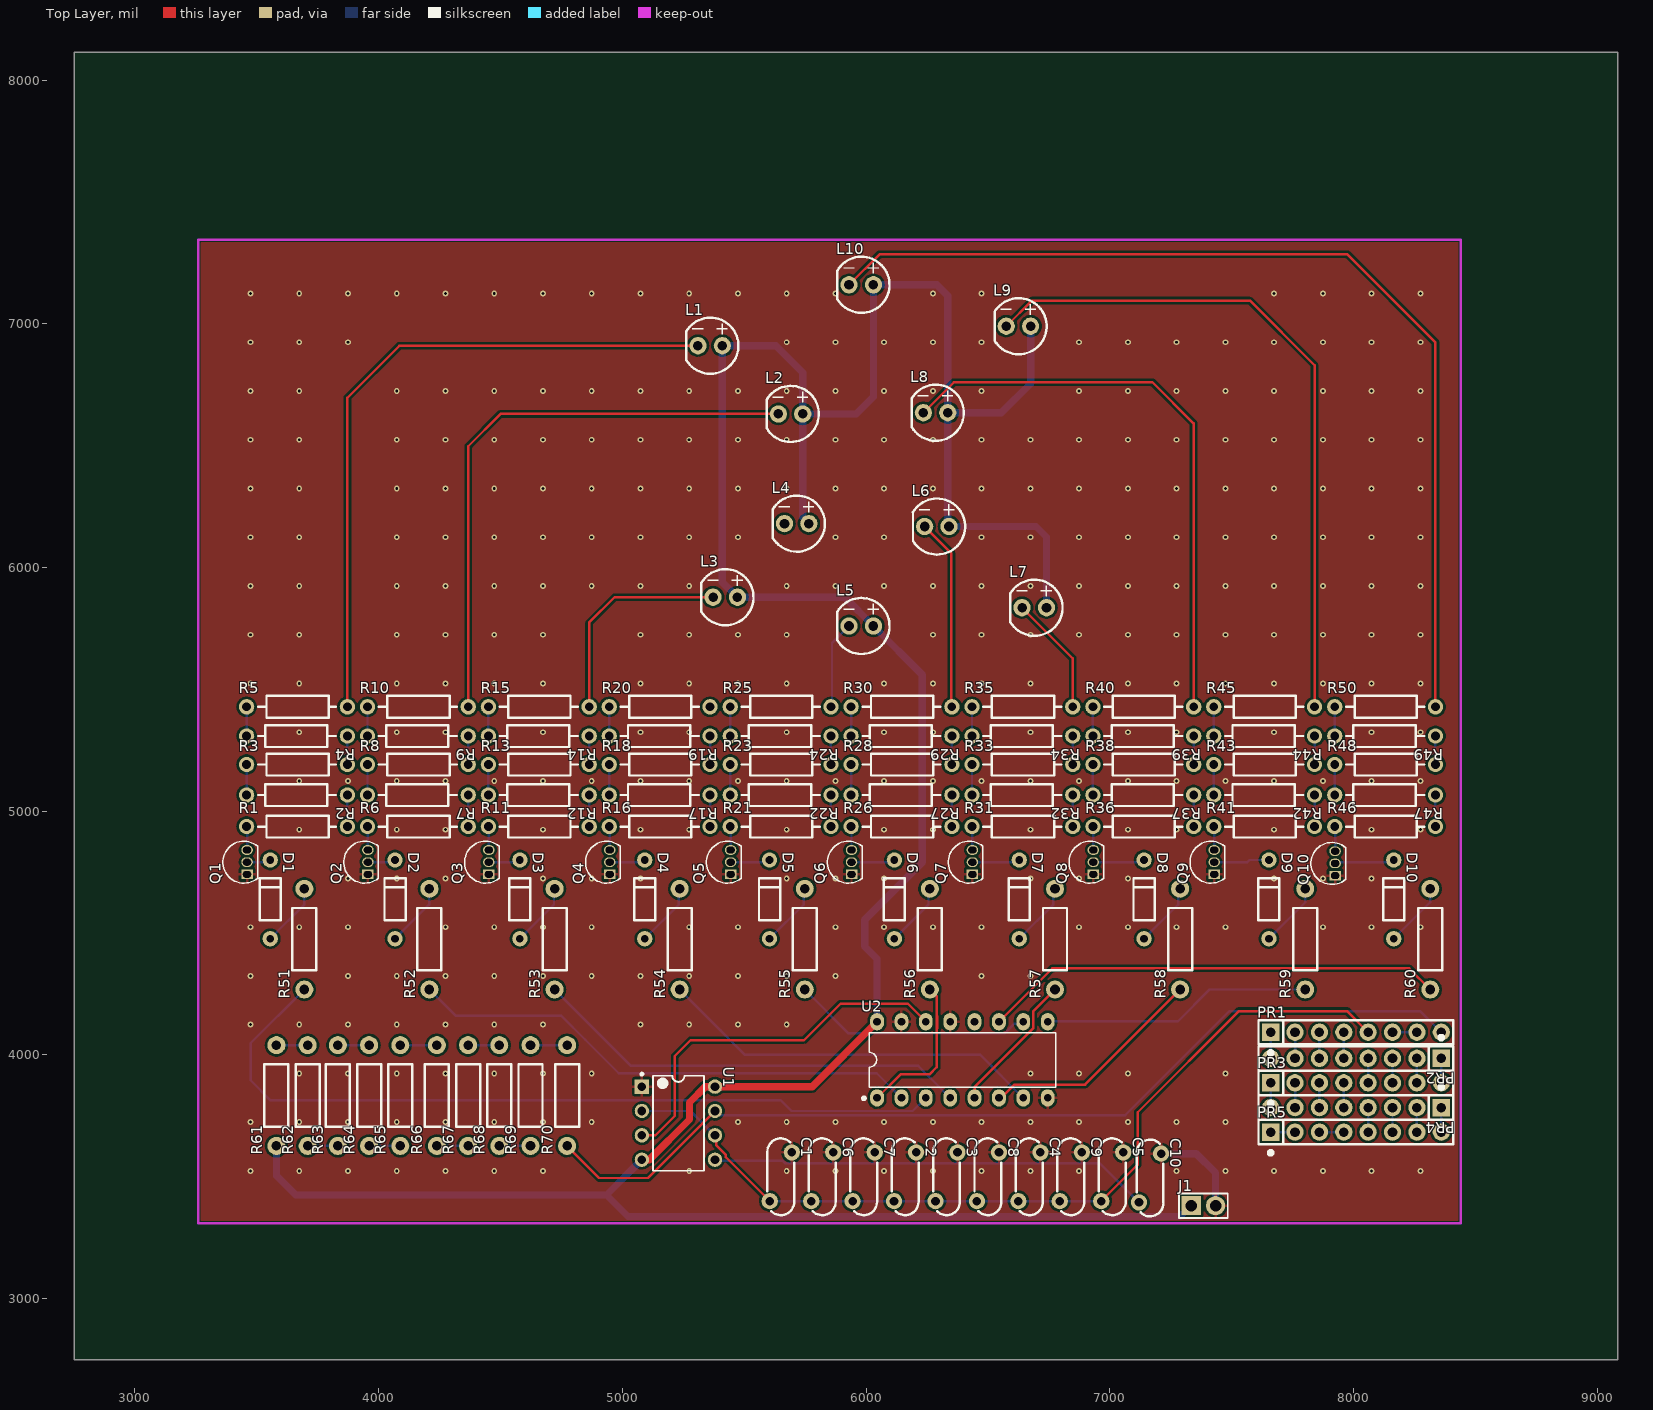
[diagram p0: Top Layer view]
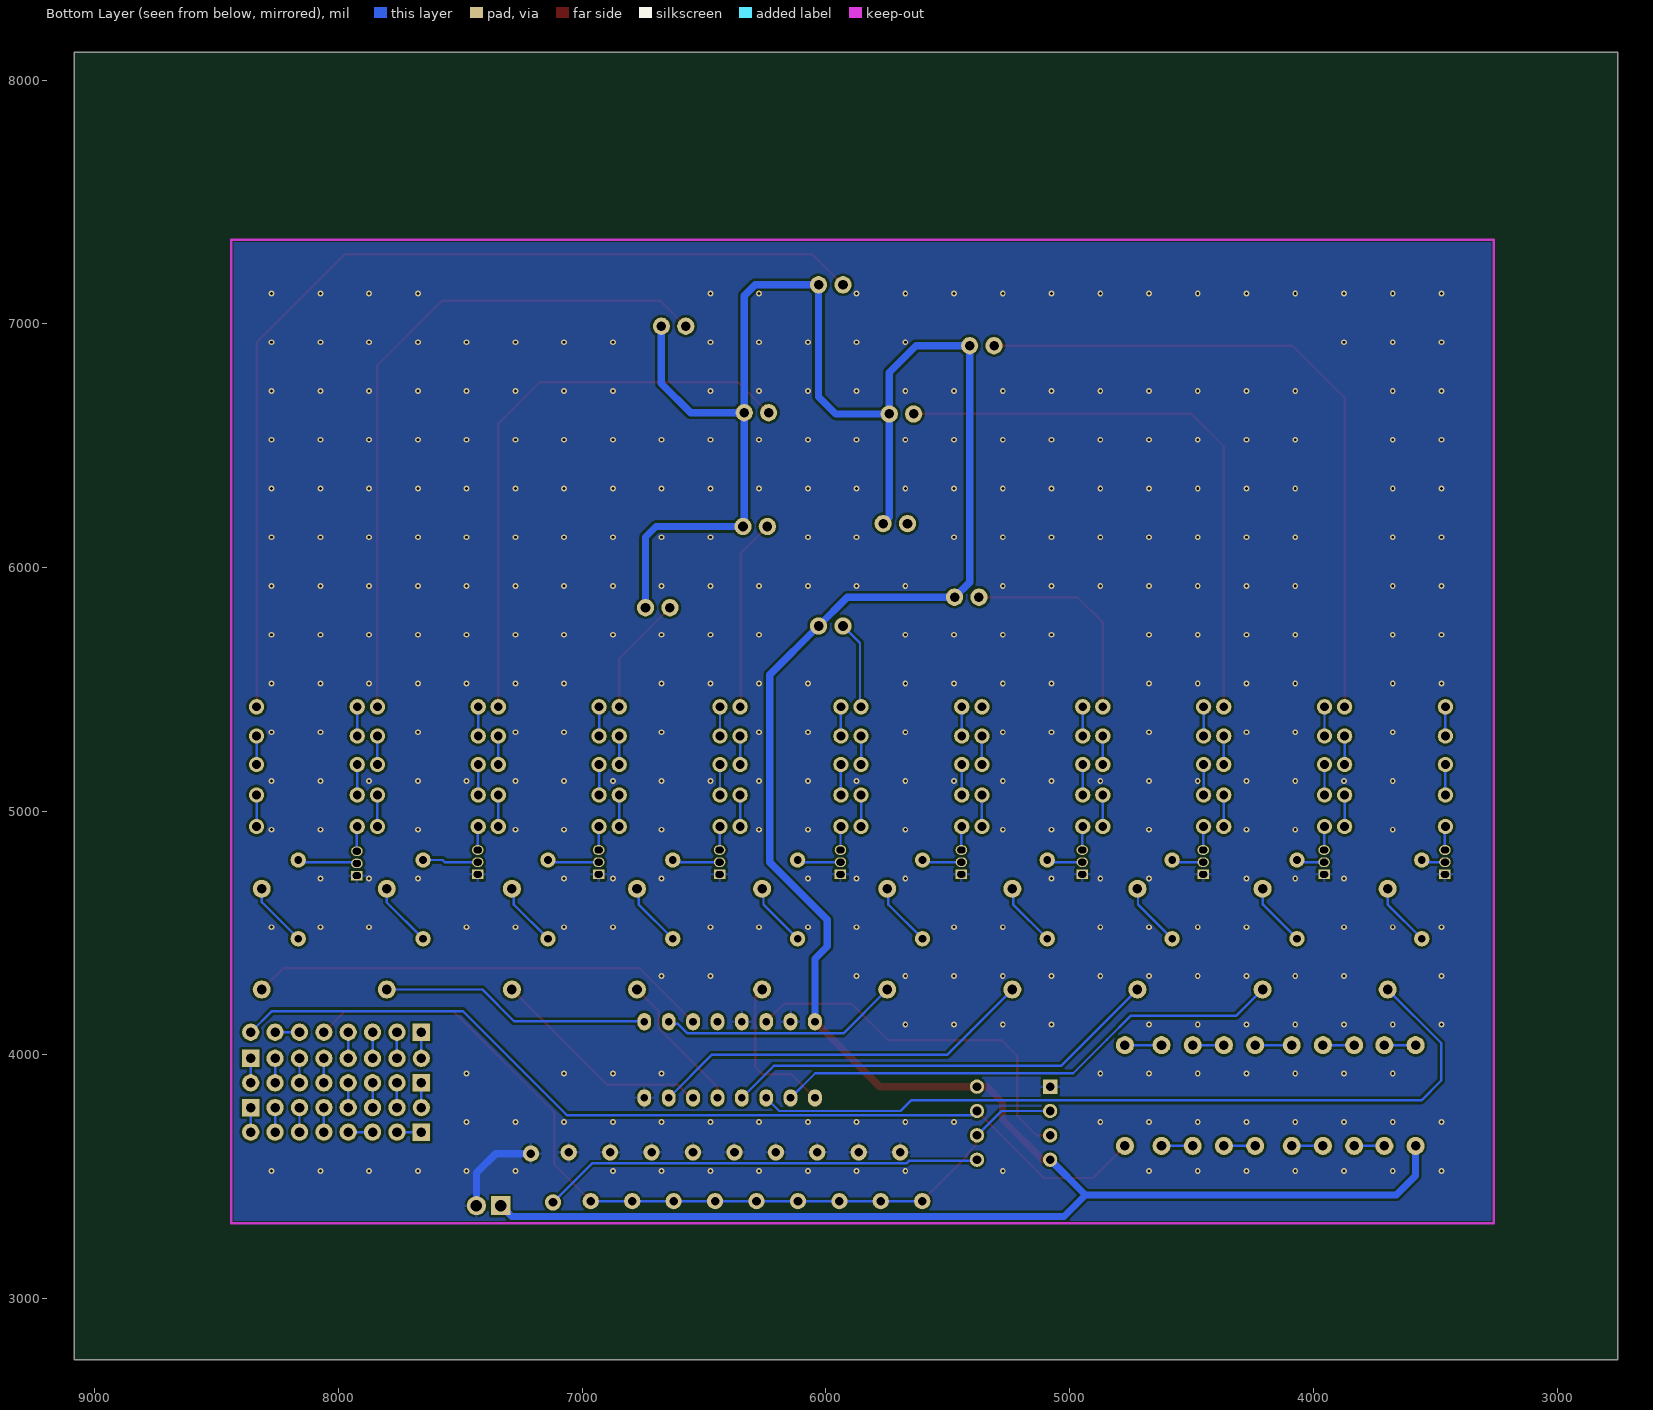
[diagram p1: Bottom Layer view, seen from below]
# Altium PCB MISC52150.pcbdoc
Units mil, origin at the board's own origin, x right, y up, seen from the top; angles counter-clockwise.
Board outline 6335 x 5365 mil, 2 copper layers (Top Layer, Bottom Layer), stack 62.206 mil thick; 118 components, 124 nets, 296 pads, 358 vias.

## Layer stack, top to bottom
Top Solder Mask Layer: solder mask 0.394, Dk 3.3
Top Layer: signal copper 1.379
Dielectric1: surface 59.449, FR4, Dk 4.5
Bottom Layer: signal copper 1.378
Bottom Solder Mask Layer: solder mask 0.394, Dk 3.3

## Board outline
9085,2750 2750,2750 2750,8115 9085,8115

## Design rules (kind name [scope] priority, off if disabled: settings)
BoardOutlineClearance copperThickness2oz_1 [All] p2 off: genericclearance=7.99 ignorepadtopadclearanceinfootprint=FALSE except(0: Arc-SplitContinuation Track-SplitContinuation SMDPad-SplitContinuation THPad-SplitContinuation Via-SplitContinuation Fill-SplitContinuation Region-SplitContinuation Poly-SplitContinuation Text-SplitContinuation Hole-SplitContinuation; 5.98: Arc-CutoutEdge SMDPad-CutoutEdge THPad-CutoutEdge Via-CutoutEdge Fill-CutoutEdge Region-CutoutEdge Text-CutoutEdge; 6.93: Hole-OutlineEdge Hole-CutoutEdge; 10: Poly-OutlineEdge Poly-CutoutEdge; 11.81: Arc-OutlineEdge Track-OutlineEdge SMDPad-OutlineEdge THPad-OutlineEdge Via-OutlineEdge Fill-OutlineEdge Region-OutlineEdge Text-OutlineEdge Track-CutoutEdge)
BoardOutlineClearance copperThickness1oz_1 [All] p4: genericclearance=4.02 ignorepadtopadclearanceinfootprint=FALSE except(0: Arc-SplitContinuation Track-SplitContinuation SMDPad-SplitContinuation THPad-SplitContinuation Via-SplitContinuation Fill-SplitContinuation Region-SplitContinuation Poly-SplitContinuation Text-SplitContinuation Hole-SplitContinuation; 6: SMDPad-CutoutEdge THPad-CutoutEdge Via-CutoutEdge Fill-CutoutEdge Region-CutoutEdge Text-CutoutEdge; 6.93: Hole-OutlineEdge Hole-CutoutEdge; 10: Poly-OutlineEdge Poly-CutoutEdge; 11.8: Arc-OutlineEdge Track-OutlineEdge SMDPad-OutlineEdge THPad-OutlineEdge Via-OutlineEdge Fill-OutlineEdge Region-OutlineEdge Text-OutlineEdge; 11.81: Arc-CutoutEdge Track-CutoutEdge)
Clearance copperThickness2oz [All] p1 off: gap=7.99 ignorepadtopadclearanceinfootprint=FALSE except(5.98: SMDPad-Track SMDPad-SMDPad THPad-Track SMDPad-THPad THPad-THPad Track-Via SMDPad-Via THPad-Via Via-Via Fill-Track Region-Track Fill-SMDPad Region-SMDPad Fill-THPad Region-THPad Fill-Via Region-Via Fill-Fill Fill-Region Region-Region Arc-Track Arc-SMDPad Arc-THPad Arc-Via Fill-Arc Region-Arc Arc-Arc Text-Track SMDPad-Text Text-THPad Text-Via Fill-Text Region-Text Arc-Text Text-Text; 6.93: Hole-Track Hole-SMDPad Hole-THPad Hole-Via Fill-Hole Region-Hole Hole-Arc Hole-Text; 10: Poly-Track Poly-SMDPad Poly-THPad Poly-Via Poly-Fill Poly-Region Poly-Poly Poly-Arc Poly-Text Poly-Hole)
Clearance copperThickness1oz [All] p3: gap=4.02 ignorepadtopadclearanceinfootprint=FALSE except(5.98: SMDPad-Track SMDPad-SMDPad THPad-Track SMDPad-THPad THPad-THPad Track-Via SMDPad-Via THPad-Via Via-Via Fill-Track Region-Track Fill-SMDPad Region-SMDPad Fill-THPad Region-THPad Fill-Via Region-Via Fill-Fill Fill-Region Region-Region; 6: Arc-Track Arc-SMDPad Arc-THPad Arc-Via Fill-Arc Region-Arc Arc-Arc Text-Track SMDPad-Text Text-THPad Text-Via Fill-Text Region-Text Arc-Text Text-Text; 6.93: Hole-Track Hole-SMDPad Hole-THPad Hole-Via Fill-Hole Region-Hole Hole-Arc Hole-Text; 10: Poly-Track Poly-SMDPad Poly-THPad Poly-Via Poly-Fill Poly-Region Poly-Poly Poly-Arc Poly-Text Poly-Hole)
DiffPairsRouting differentialPair [All] p1: maxlimit=6 minlimit=6 mostfreqgap=6 toplayer_minwidth=5 toplayer_prefwidth=10 toplayer_maxwidth=100 toplayer_mingap=6 toplayer_prefgap=6 toplayer_maxgap=6 bottomlayer_minwidth=5 bottomlayer_prefwidth=10 bottomlayer_maxwidth=100 bottomlayer_mingap=6 bottomlayer_prefgap=6 bottomlayer_maxgap=6 maxuncoupledlength=10
HoleToHoleClearance otherClearance [All] p1: gap=11.81 allowstackedmicrovias=TRUE
Length netLength [All] p1: minlimit=0 maxlimit=0
MatchedLengths netLengthTolerance [All] p1: tolerance=1000
PasteMaskExpansion pasteMaskExpansion [All] p1: expansion=0
PlaneConnect innerPlane [All] p1: planeconnectstyle=Relief reliefexpansion=20 reliefentries=4 reliefconductorwidth=10 reliefairgap=10
PolygonConnect copperRegion [(InNet('GND'))] p1: connectstyle=Relief reliefconductorwidth=10 reliefentries=4 polygonreliefangle="90 Angle" airgapwidth=10 via.connectstyle=Relief via.reliefconductorwidth=10 via.reliefentries=4 via.polygonreliefangle="90 Angle" via.airgapwidth=10
RoutingVias viaSize [All] p1: holewidth=12.01 width=24.02 viastyle="Through Hole" minholewidth=11.81 minwidth=19.68 maxholewidth=248.03 maxwidth=393.7
SolderMaskExpansion solderMaskExpansion [IsVia] p1: expansion=-1000 istentingtop=TRUE
SolderMaskExpansion solderMaskExpansion [All] p2: expansion=2 istentingtop=FALSE
Width copperThickness2oz_2 [All] p1 off: maxlimit=100 minlimit=8 preferedwidth=10
Width copperThickness1oz_2 [All] p2: maxlimit=100 minlimit=5 preferedwidth=10

## Components (designator, comment, footprint, x,y, rotation, side; value= is the part's Value field where it differs from the comment)
C1 "10nF" CAP-TH_L8.0-W2.8-P5.08-D0.6 5650,3500 r270 top
C2 "10nF" CAP-TH_L8.0-W2.8-P5.08-D0.6 6160,3500 r270 top
C3 "10nF" CAP-TH_L8.0-W2.8-P5.08-D0.6 6330,3500 r270 top
C4 "10nF" CAP-TH_L8.0-W2.8-P5.08-D0.6 6670,3500 r270 top
C5 "10nF" CAP-TH_L8.0-W2.8-P5.08-D0.6 7010,3500 r270 top
C6 "10nF" CAP-TH_L8.0-W2.8-P5.08-D0.6 5820,3500 r270 top
C7 "10nF" CAP-TH_L8.0-W2.8-P5.08-D0.6 5990,3500 r270 top
C8 "10nF" CAP-TH_L8.0-W2.8-P5.08-D0.6 6500,3500 r270 top
C9 "10nF" CAP-TH_L8.0-W2.8-P5.08-D0.6 6840,3500 r270 top
C10 "10nF" CAP-TH_L8.0-W2.8-P5.08-D0.6 7165,3495 r270 top
D1 "1N4148TR" DO-35_BD2.0-L4.2-P8.20-D0.5-RD 3555,4638.39 r270 top
D2 "1N4148TR" DO-35_BD2.0-L4.2-P8.20-D0.5-RD 4067.22,4638.39 r270 top
D3 "1N4148TR" DO-35_BD2.0-L4.2-P8.20-D0.5-RD 4579.44,4638.39 r270 top
D4 "1N4148TR" DO-35_BD2.0-L4.2-P8.20-D0.5-RD 5091.67,4638.39 r270 top
D5 "1N4148TR" DO-35_BD2.0-L4.2-P8.20-D0.5-RD 5603.89,4638.39 r270 top
D6 "1N4148TR" DO-35_BD2.0-L4.2-P8.20-D0.5-RD 6116.11,4638.39 r270 top
D7 "1N4148TR" DO-35_BD2.0-L4.2-P8.20-D0.5-RD 6628.33,4638.39 r270 top
D8 "1N4148TR" DO-35_BD2.0-L4.2-P8.20-D0.5-RD 7140.56,4638.39 r270 top
D9 "1N4148TR" DO-35_BD2.0-L4.2-P8.20-D0.5-RD 7652.78,4638.39 r270 top
D10 "1N4148TR" DO-35_BD2.0-L4.2-P8.20-D0.5-RD 8165,4638.39 r270 top
J1 "PZ254V-11-02P" HDR-TH_2P-P2.54-V-M 7383.93,3381.56 r0 top
L1 "XL-502SURD" LED-TH_BD5.9-P2.54-RD_RED 5360,6910 r0 top
L2 "XL-502SURD" LED-TH_BD5.9-P2.54-RD_RED 5690,6630 r0 top
L3 "XL-502SURD" LED-TH_BD5.9-P2.54-RD_RED 5421.98,5878.08 r0 top
L4 "XL-502SURD" LED-TH_BD5.9-P2.54-RD_RED 5715,6180 r0 top
L5 "XL-502SURD" LED-TH_BD5.9-P2.54-RD_RED 5980,5760 r0 top
L6 "XL-502SURD" LED-TH_BD5.9-P2.54-RD_RED 6290.18,6168.08 r0 top
L7 "XL-502SURD" LED-TH_BD5.9-P2.54-RD_RED 6690,5835 r0 top
L8 "XL-502SURD" LED-TH_BD5.9-P2.54-RD_RED 6285,6635 r0 top
L9 "XL-502SURD" LED-TH_BD5.9-P2.54-RD_RED 6625,6990 r0 top
L10 "XL-502SURD" LED-TH_BD5.9-P2.54-RD_RED 5980,7160 r0 top
PR1 "10kΩ" RES-ARRAY-TH_8P-L20.3-W2.5-P2.54 8010,4093.09 r0 top
PR2 "10kΩ" RES-ARRAY-TH_8P-L20.3-W2.5-P2.54 8010,3986.11 r180 top
PR3 "10kΩ" RES-ARRAY-TH_8P-L20.3-W2.5-P2.54 8010,3885.62 r0 top
PR4 "10kΩ" RES-ARRAY-TH_8P-L20.3-W2.5-P2.54 8010,3783.65 r180 top
PR5 "10kΩ" RES-ARRAY-TH_8P-L20.3-W2.5-P2.54 8010,3683.16 r0 top
Q1 "S8050" TO-92-3_L4.5-W3.5-P1.27-L 3459.84,4790.8 r90 top
Q2 "S8050" TO-92-3_L4.5-W3.5-P1.27-L 3955.91,4790.8 r90 top
Q3 "S8050" TO-92-3_L4.5-W3.5-P1.27-L 4451.98,4790.8 r90 top
Q4 "S8050" TO-92-3_L4.5-W3.5-P1.27-L 4948.05,4790.8 r90 top
Q5 "S8050" TO-92-3_L4.5-W3.5-P1.27-L 5444.11,4790.8 r90 top
Q6 "S8050" TO-92-3_L4.5-W3.5-P1.27-L 5940.18,4790.8 r90 top
Q7 "S8050" TO-92-3_L4.5-W3.5-P1.27-L 6436.25,4790.8 r90 top
Q8 "S8050" TO-92-3_L4.5-W3.5-P1.27-L 6932.31,4790.8 r90 top
Q9 "S8050" TO-92-3_L4.5-W3.5-P1.27-L 7428.38,4790.8 r90 top
Q10 "S8050" TO-92-3_L4.5-W3.5-P1.27-L 7924.45,4785.8 r90 top
R1 "100Ω" RES-TH_BD2.2-L6.5-P10.50-D0.6 3664.84,4937.09 r0 top
R2 "100Ω" RES-TH_BD2.2-L6.5-P10.50-D0.6 3664.84,5066.43 r180 top
R3 "100Ω" RES-TH_BD2.2-L6.5-P10.50-D0.6 3664.84,5191.55 r0 top
R4 "100Ω" RES-TH_BD2.2-L6.5-P10.50-D0.6 3664.84,5308.56 r180 top
R5 "100Ω" RES-TH_BD2.2-L6.5-P10.50-D0.6 3664.84,5428.24 r0 top
R6 "100Ω" RES-TH_BD2.2-L6.5-P10.50-D0.6 4160.91,4937.09 r0 top
R7 "100Ω" RES-TH_BD2.2-L6.5-P10.50-D0.6 4160.91,5066.43 r180 top
R8 "100Ω" RES-TH_BD2.2-L6.5-P10.50-D0.6 4160.91,5191.55 r0 top
R9 "100Ω" RES-TH_BD2.2-L6.5-P10.50-D0.6 4160.91,5308.56 r180 top
R10 "100Ω" RES-TH_BD2.2-L6.5-P10.50-D0.6 4160.91,5428.24 r0 top
R11 "100Ω" RES-TH_BD2.2-L6.5-P10.50-D0.6 4656.98,4937.09 r0 top
R12 "100Ω" RES-TH_BD2.2-L6.5-P10.50-D0.6 4656.98,5066.43 r180 top
R13 "100Ω" RES-TH_BD2.2-L6.5-P10.50-D0.6 4656.98,5191.55 r0 top
R14 "100Ω" RES-TH_BD2.2-L6.5-P10.50-D0.6 4656.98,5308.56 r180 top
R15 "100Ω" RES-TH_BD2.2-L6.5-P10.50-D0.6 4656.98,5428.24 r0 top
R16 "100Ω" RES-TH_BD2.2-L6.5-P10.50-D0.6 5153.05,4937.09 r0 top
R17 "100Ω" RES-TH_BD2.2-L6.5-P10.50-D0.6 5153.05,5066.43 r180 top
R18 "100Ω" RES-TH_BD2.2-L6.5-P10.50-D0.6 5153.05,5191.55 r0 top
R19 "100Ω" RES-TH_BD2.2-L6.5-P10.50-D0.6 5153.05,5308.56 r180 top
R20 "100Ω" RES-TH_BD2.2-L6.5-P10.50-D0.6 5153.05,5428.24 r0 top
R21 "100Ω" RES-TH_BD2.2-L6.5-P10.50-D0.6 5649.11,4937.09 r0 top
R22 "100Ω" RES-TH_BD2.2-L6.5-P10.50-D0.6 5649.11,5066.43 r180 top
R23 "100Ω" RES-TH_BD2.2-L6.5-P10.50-D0.6 5649.11,5191.55 r0 top
R24 "100Ω" RES-TH_BD2.2-L6.5-P10.50-D0.6 5649.11,5308.56 r180 top
R25 "100Ω" RES-TH_BD2.2-L6.5-P10.50-D0.6 5649.11,5428.24 r0 top
R26 "100Ω" RES-TH_BD2.2-L6.5-P10.50-D0.6 6145.18,4937.09 r0 top
R27 "100Ω" RES-TH_BD2.2-L6.5-P10.50-D0.6 6145.18,5066.43 r180 top
R28 "100Ω" RES-TH_BD2.2-L6.5-P10.50-D0.6 6145.18,5191.55 r0 top
R29 "100Ω" RES-TH_BD2.2-L6.5-P10.50-D0.6 6145.18,5308.56 r180 top
R30 "100Ω" RES-TH_BD2.2-L6.5-P10.50-D0.6 6145.18,5428.24 r0 top
R31 "100Ω" RES-TH_BD2.2-L6.5-P10.50-D0.6 6641.25,4937.09 r0 top
R32 "100Ω" RES-TH_BD2.2-L6.5-P10.50-D0.6 6641.25,5066.43 r180 top
R33 "100Ω" RES-TH_BD2.2-L6.5-P10.50-D0.6 6641.25,5191.55 r0 top
R34 "100Ω" RES-TH_BD2.2-L6.5-P10.50-D0.6 6641.25,5308.56 r180 top
R35 "100Ω" RES-TH_BD2.2-L6.5-P10.50-D0.6 6641.25,5428.24 r0 top
R36 "100Ω" RES-TH_BD2.2-L6.5-P10.50-D0.6 7137.31,4937.09 r0 top
R37 "100Ω" RES-TH_BD2.2-L6.5-P10.50-D0.6 7137.31,5066.43 r180 top
R38 "100Ω" RES-TH_BD2.2-L6.5-P10.50-D0.6 7137.31,5191.55 r0 top
R39 "100Ω" RES-TH_BD2.2-L6.5-P10.50-D0.6 7137.31,5308.56 r180 top
R40 "100Ω" RES-TH_BD2.2-L6.5-P10.50-D0.6 7137.31,5428.24 r0 top
R41 "100Ω" RES-TH_BD2.2-L6.5-P10.50-D0.6 7633.38,4937.09 r0 top
R42 "100Ω" RES-TH_BD2.2-L6.5-P10.50-D0.6 7633.38,5066.43 r180 top
R43 "100Ω" RES-TH_BD2.2-L6.5-P10.50-D0.6 7633.38,5191.55 r0 top
R44 "100Ω" RES-TH_BD2.2-L6.5-P10.50-D0.6 7633.38,5308.56 r180 top
R45 "100Ω" RES-TH_BD2.2-L6.5-P10.50-D0.6 7633.38,5428.24 r0 top
R46 "100Ω" RES-TH_BD2.2-L6.5-P10.50-D0.6 8129.45,4937.09 r0 top
R47 "100Ω" RES-TH_BD2.2-L6.5-P10.50-D0.6 8129.45,5066.43 r180 top
R48 "100Ω" RES-TH_BD2.2-L6.5-P10.50-D0.6 8129.45,5191.55 r0 top
R49 "100Ω" RES-TH_BD2.2-L6.5-P10.50-D0.6 8129.45,5308.56 r180 top
R50 "100Ω" RES-TH_BD2.2-L6.5-P10.50-D0.6 8129.45,5428.24 r0 top
R51 "1kΩ" RES-TH_BD2.5-L6.5-P10.50-D0.6 3695,4475 r90 top
R52 "1kΩ" RES-TH_BD2.5-L6.5-P10.50-D0.6 4208.33,4475 r90 top
R53 "1kΩ" RES-TH_BD2.5-L6.5-P10.50-D0.6 4721.67,4475 r90 top
R54 "1kΩ" RES-TH_BD2.5-L6.5-P10.50-D0.6 5235,4475 r90 top
R55 "1kΩ" RES-TH_BD2.5-L6.5-P10.50-D0.6 5748.33,4475 r90 top
R56 "1kΩ" RES-TH_BD2.5-L6.5-P10.50-D0.6 6261.67,4475 r90 top
R57 "1kΩ" RES-TH_BD2.5-L6.5-P10.50-D0.6 6775,4475 r90 top
R58 "1kΩ" RES-TH_BD2.5-L6.5-P10.50-D0.6 7288.33,4475 r90 top
R59 "1kΩ" RES-TH_BD2.5-L6.5-P10.50-D0.6 7801.67,4475 r90 top
R60 "1kΩ" RES-TH_BD2.5-L6.5-P10.50-D0.6 8315,4475 r90 top
R61 "1kΩ" RES-TH_BD2.5-L6.5-P10.50-D0.6 3580.49,3833.38 r90 top
R62 "1kΩ" RES-TH_BD2.5-L6.5-P10.50-D0.6 3708.6,3833.38 r90 top
R63 "1kΩ" RES-TH_BD2.5-L6.5-P10.50-D0.6 3832.5,3833.38 r90 top
R64 "1kΩ" RES-TH_BD2.5-L6.5-P10.50-D0.6 3960.61,3833.38 r90 top
R65 "1kΩ" RES-TH_BD2.5-L6.5-P10.50-D0.6 4088.72,3833.38 r90 top
R66 "1kΩ" RES-TH_BD2.5-L6.5-P10.50-D0.6 4238.72,3833.38 r90 top
R67 "1kΩ" RES-TH_BD2.5-L6.5-P10.50-D0.6 4366.83,3833.38 r90 top
R68 "1kΩ" RES-TH_BD2.5-L6.5-P10.50-D0.6 4494.94,3833.38 r90 top
R69 "1kΩ" RES-TH_BD2.5-L6.5-P10.50-D0.6 4623.05,3833.38 r90 top
R70 "1kΩ" RES-TH_BD2.5-L6.5-P10.50-D0.6 4773.05,3833.38 r90 top
U1 "NE555P" DIP-8_L9.8-W6.6-P2.54-LS7.6-BL 5230,3720 r270 top
U2 "CD4017CN" PDIP-16_L19.3-W6.4-P2.54-LS7.94-BL 6395,3980 r0 top

## Footprints (in the part's own frame and the unit in brackets; to place one, negate y for a bottom-side part, rotate by r counter-clockwise, add the part's x,y. Pads: shape width x height; smd on the part's side, far side on the other; paste and mask are expansions set on the pad)
CAP-TH_L8.0-W2.8-P5.08-D0.6 [mm]
  round 1.7 hole 0.9 paste+0 mask+0.05: 1(-2.54,1.15) 2(2.54,-1.15)
  silkscreen extent -4,-1.4 4,1.4
DIP-8_L9.8-W6.6-P2.54-LS7.6-BL [mm]
  rect 1.5x1.5 hole 0.9: 1(-3.81,-3.81)
  round 1.5 hole 0.9: 2(-1.27,-3.81) 3(1.27,-3.81) 4(3.81,-3.81) 5(3.81,3.81) 6(1.27,3.81) 7(-1.27,3.81) 8(-3.81,3.81)
  silkscreen extent -5.23,-3.93 4.96,2.65
DO-35_BD2.0-L4.2-P8.20-D0.5-RD [mm]
  round 1.6 hole 0.8: 1(-4.1,0) 2(4.1,0)
  silkscreen extent -2.2,-1.1 2.2,1.1
HDR-TH_2P-P2.54-V-M [mm]
  rect 2x2 hole 1.2: 1(-1.27,0)
  round 2 hole 1.2: 2(1.27,0)
  silkscreen extent -2.54,-1.27 2.54,1.27
LED-TH_BD5.9-P2.54-RD_RED [mm]
  round 1.8 hole 1 paste+0 mask+0.05: 1(-1.27,0) 2(1.27,0)
  silkscreen extent -2.49,-2.92 2.94,2.92
PDIP-16_L19.3-W6.4-P2.54-LS7.94-BL [mm]
  oval 1.44x1.8 hole 0.8: 1(-8.89,-3.97) 2(-6.35,-3.97) 3(-3.81,-3.97) 4(-1.27,-3.97) 5(1.27,-3.97) 6(3.81,-3.97) 7(6.35,-3.97) 8(8.89,-3.97) 9(8.89,3.97) 10(6.35,3.97) 11(3.81,3.97) 12(1.27,3.97) 13(-1.27,3.97) 14(-3.81,3.97) 15(-6.35,3.97) 16(-8.89,3.97)
  silkscreen extent -10.41,-4.17 9.73,2.84
RES-ARRAY-TH_8P-L20.3-W2.5-P2.54 [mm]
  rect 1.8x1.8 hole 1: 1(-8.89,0)
  round 1.8 hole 1: 2(-6.35,0) 3(-3.81,0) 4(-1.27,0) 5(1.27,0) 6(3.81,0) 7(6.35,0) 8(8.89,0)
  silkscreen extent -10.16,-2.36 10.16,1.27
RES-TH_BD2.2-L6.5-P10.50-D0.6 [mm]
  round 1.6 hole 0.914: 1(-5.25,0) 2(5.25,0)
  silkscreen extent -4.06,-1.14 4.06,1.14
RES-TH_BD2.5-L6.5-P10.50-D0.6 [mil]
  round 74 hole 39.37: 1(-206.69,0) 2(206.69,0)
  silkscreen extent -128,-49 128,49
TO-92-3_L4.5-W3.5-P1.27-L [mm]
  rect 1x1.2 hole 0.7 slot 0.85 at 90 deg: 1(-1.27,0)
  oval 1x1.2 hole 0.7 slot 0.85 at 90 deg: 2(0,0) 3(1.27,0)
  silkscreen extent -2.19,-1.1 2.19,2.52

## Via types
v1: diameter 24.02, hole 12, Top Layer to Bottom Layer, 358 vias

## Nets (pads, with @x,y where several pads share a name; then routed paths per layer and width w, separated by ;. In a path a pad name is that pad's centre, name@x,y a point inside that pad or via, vN(x,y) a via of type N, cw(c..) or ccw(c..) an arc to the next point about the centre after c; other vN are vias at no path point)
$1N509: U1.3 U2.14 | length 1562.7
  Top Layer w10: U1.3 5135,3670 5215,3750 5215,3995 5280,4060 5745,4060 5895,4210 6171.3,4210 U2.14
$1N552: C10.2 U1.5 | length 1811.3
  Bottom Layer w10: U1.5 5389.72,3565 5659.72,3565 5669.72,3555 6959.72,3555 C10.2
$1N1039: R60.1 U2.11 | length 1896.5
  Top Layer w10: U2.11 6763.7,4355 8228.31,4355 R60.1
$1N1041: R59.1 U2.9 | length 1110.6
  Bottom Layer w10: U2.9 6761.67,4138.31 7279.71,4138.31 7409.71,4268.31 R59.1
$1N1043: R58.1 U2.6 | length 927.5
  Top Layer w10: U2.6 6553.73,3823.7 6608.34,3878.31 6898.34,3878.31 R58.1
$1N1045: R57.1 U2.5 | length 581.3
  Top Layer w10: U2.5 6445,3868.31 6685,4108.31 6685,4178.31 R57.1
$1N1047: R56.1 U2.1 | length 692.2
  Top Layer w10: R56.1 6290,4239.98 6290,4159.98 ; U2.1@6051.67,3830.37 6051.67,3828.31 U2.1 U2.1@6051.67,3830.37 ; U2.1@6051.67,3830.37 6141.3,3920 6260,3920 6290,3950 6290,4106.64 ; 6290,4106.64 6290,4159.98 ; 6290,4106.64 6291.67,4108.31 6291.67,4158.31 6290,4159.98
$1N1049: R55.1 U2.10 | length 989.6
  Bottom Layer w10: R55.1 5928.33,4088.31 6568.33,4088.31 6608.33,4128.31 6628.33,4128.31 U2.10
$1N1051: R54.1 U2.7 | length 1594.2
  Bottom Layer w10: R54.1 5402.89,4100.42 5503.31,4000 6468.7,4000 U2.7
$1N1053: R53.1 U2.4 | length 1807.5
  Bottom Layer w10: R53.1 4912.26,4077.72 5034.98,3955 6213.7,3955 U2.4
$1N1055: R51.1 U2.3 | length 3308.5
  Bottom Layer w10: R51.1 3475,4048.31 3475,3895 3556.3,3813.7 5650.32,3813.7 5694.02,3770 6191.3,3770 U2.3
$1N1057: R52.1 U2.2 | length 2120.8
  Bottom Layer w10: R52.1 4316.64,4160 4750,4160 4847.69,4062.31 4985,3925 6043.7,3925 U2.2
$1N1689: R4.2 R5.1 | length 119.7
  Bottom Layer w10: R4.2@3458.15,5308.56 R5.1
$1N1693: R3.2 R4.1 | length 117
  Bottom Layer w10: R3.2 R4.1
$1N1698: R2.2 R3.1 | length 125.1
  Bottom Layer w10: R2.2@3458.15,5066.43 R3.1
$1N1703: R1.2 R2.1 | length 129.3
  Bottom Layer w10: R1.2 R2.1
$1N1886: R6.2 R7.1 | length 129.3
  Bottom Layer w10: R6.2 R7.1
$1N1888: R8.2 R9.1 | length 117
  Bottom Layer w10: R8.2 R9.1
$1N1890: R7.2 R8.1 | length 125.1
  Bottom Layer w10: R7.2 R8.1
$1N1892: R9.2 R10.1 | length 119.7
  Bottom Layer w10: R9.2 R10.1
$1N2074: R11.2 R12.1 | length 129.3
  Bottom Layer w10: R11.2 R12.1
$1N2076: R13.2 R14.1 | length 117
  Bottom Layer w10: R13.2 R14.1
$1N2078: R12.2 R13.1 | length 125.1
  Bottom Layer w10: R12.2 R13.1
$1N2080: R14.2 R15.1 | length 119.7
  Bottom Layer w10: R14.2 R15.1
$1N2826: R16.2 R17.1 | length 129.3
  Bottom Layer w10: R16.2 R17.1
$1N2828: R18.2 R19.1 | length 117
  Bottom Layer w10: R18.2 R19.1
$1N2830: R17.2 R18.1 | length 125.1
  Bottom Layer w10: R17.2@4946.35,5066.43 R18.1@4946.35,5191.54
$1N2832: R19.2 R20.1 | length 119.7
  Bottom Layer w10: R19.2@4946.35,5308.56 R20.1@4946.35,5428.24
$1N3014: R21.2 R22.1 | length 129.3
  Bottom Layer w10: R21.2 R22.1
$1N3016: R23.2 R24.1 | length 117
  Bottom Layer w10: R23.2 R24.1
$1N3018: R22.2 R23.1 | length 125.1
  Bottom Layer w10: R22.2 R23.1
$1N3020: R24.2 R25.1 | length 119.7
  Bottom Layer w10: R24.2 R25.1
$1N4862: R32.2 R33.1 | length 125.1
  Bottom Layer w10: R32.2@6434.55,5066.43 R33.1@6434.55,5191.54
$1N4864: R33.2 R34.1 | length 117
  Bottom Layer w10: R33.2 R34.1
$1N4866: R31.2 R32.1 | length 129.3
  Bottom Layer w10: R31.2 R32.1
$1N4868: R34.2 R35.1 | length 119.7
  Bottom Layer w10: R34.2@6434.55,5308.56 R35.1@6434.55,5428.24
$1N4870: R26.2 R27.1 | length 129.3
  Bottom Layer w10: R26.2 R27.1
$1N4872: R27.2 R28.1 | length 125.1
  Bottom Layer w10: R27.2 R28.1
$1N4874: R28.2 R29.1 | length 117
  Bottom Layer w10: R28.2 R29.1
$1N4876: R29.2 R30.1 | length 119.7
  Bottom Layer w10: R29.2 R30.1
$1N4878: R37.2 R38.1 | length 125.1
  Bottom Layer w10: R37.2 R38.1
$1N4880: R39.2 R40.1 | length 119.7
  Bottom Layer w10: R39.2 R40.1
$1N4882: R36.2 R37.1 | length 129.3
  Bottom Layer w10: R36.2 R37.1
$1N4884: R38.2 R39.1 | length 117
  Bottom Layer w10: R38.2 R39.1
$1N4886: R47.2 R48.1 | length 125.1
  Bottom Layer w10: R47.2 R48.1
$1N4888: R48.2 R49.1 | length 117
  Bottom Layer w10: R48.2 R49.1
$1N4890: R46.2 R47.1 | length 129.3
  Bottom Layer w10: R46.2 R47.1
$1N4892: R49.2 R50.1 | length 119.7
  Bottom Layer w10: R49.2 R50.1
$1N4894: R44.2 R45.1 | length 119.7
  Bottom Layer w10: R44.2 R45.1
$1N4896: R43.2 R44.1 | length 117
  Bottom Layer w10: R43.2 R44.1
$1N4898: R42.2 R43.1 | length 125.1
  Bottom Layer w10: R42.2 R43.1
$1N4900: R41.2 R42.1 | length 129.3
  Bottom Layer w10: R41.2 R42.1
$1N6278: D1.2 R51.2 | length 262.7
  Bottom Layer w10: D1.2 3695,4616.97 R51.2
$1N6282: D2.2 R52.2 | length 262.8
  Bottom Layer w10: D2.2 4207.22,4616.97 4207.22,4666.97 R52.2
$1N6287: D3.2 R53.2 | length 262.9
  Bottom Layer w10: D3.2 4719.44,4616.97 4719.44,4666.97 R53.2
$1N6292: D4.2 R54.2 | length 263.1
  Bottom Layer w10: D4.2 5231.67,4616.97 5231.67,4666.97 R54.2
$1N6297: D5.2 R55.2 | length 263.4
  Bottom Layer w10: D5.2 5743.89,4616.97 5743.89,4666.97 R55.2
$1N6302: D6.2 R56.2 | length 263.7
  Bottom Layer w10: D6.2 6256.11,4616.97 6256.11,4666.97 R56.2
$1N6307: D7.2 R57.2 | length 264.2
  Bottom Layer w10: D7.2 6768.33,4616.97 6768.33,4666.97 R57.2
$1N6312: D8.2 R58.2 | length 264.6
  Bottom Layer w10: D8.2 7280.56,4616.97 7280.56,4666.97 R58.2
$1N6317: D9.2 R59.2 | length 266.4
  Bottom Layer w10: D9.2 7801.67,4625.86 R59.2
$1N6322: D10.2 R60.2 | length 266.9
  Bottom Layer w10: D10.2 8315,4626.97 R60.2
$1N6789: Q10.3 R46.1 | length 102
  Bottom Layer w10: R46.1 7924.45,4935.4 Q10.3
$1N6799: Q9.3 R41.1 | length 97
  Bottom Layer w10: R41.1 7426.69,4932.5 7428.38,4930.8 Q9.3
$1N6801: Q8.3 R36.1 | length 96.5
  Bottom Layer w10: R36.1 6932.31,4930.8 Q8.3
$1N6803: Q7.3 R31.1 | length 96.5
  Bottom Layer w10: R31.1@6434.55,4937.09 6436.25,4930.8 Q7.3
$1N6805: Q6.3 R26.1 | length 96.5
  Bottom Layer w10: R26.1 5940.18,4930.8 Q6.3
$1N6807: Q5.3 R21.1 | length 96.5
  Bottom Layer w10: R21.1 5444.11,4930.8 Q5.3
$1N6809: Q4.3 R16.1 | length 96.5
  Bottom Layer w10: R16.1@4946.35,4937.09 4948.04,4930.8 Q4.3
$1N6811: Q3.3 R11.1 | length 97
  Bottom Layer w10: R11.1 4450.28,4932.5 4451.98,4930.8 Q3.3
$1N6813: Q2.3 R6.1 | length 96.5
  Bottom Layer w10: R6.1 3955.91,4930.8 Q2.3
$1N6815: Q1.3 R1.1 | length 96.5
  Bottom Layer w10: R1.1 3459.84,4930.8 Q1.3
$1N6819: D1.1 Q1.2 | length 98.9
  Bottom Layer w10: Q1.2 3525.99,4790.8 3535,4799.81 D1.1
$1N6827: D2.1 Q2.2 | length 115
  Bottom Layer w10: Q2.2 4038.22,4790.8 4047.22,4799.81 D2.1
$1N6833: D3.1 Q3.2 | length 131.2
  Bottom Layer w10: Q3.2 4560.43,4790.8 4569.44,4799.81 D3.1
$1N6840: D4.1 Q4.2 | length 147.4
  Bottom Layer w10: Q4.2 5072.66,4790.8 5081.67,4799.81 D4.1
$1N6847: D5.1 Q5.2 | length 163.5
  Bottom Layer w10: Q5.2 5584.88,4790.8 5593.89,4799.81 D5.1
$1N6854: D6.1 Q6.2 | length 179.7
  Bottom Layer w10: Q6.2 6107.1,4790.8 D6.1
$1N6860: D7.1 Q7.2 | length 195.8
  Bottom Layer w10: Q7.2 6619.32,4790.8 D7.1
$1N6867: D8.1 Q8.2 | length 212
  Bottom Layer w10: Q8.2 7131.55,4790.8 D8.1
$1N6874: D9.1 Q9.2 | length 228.1
  Bottom Layer w10: Q9.2 7563.77,4790.8 7572.78,4799.81 D9.1
$1N6881: D10.1 Q10.2 | length 245.4
  Bottom Layer w10: Q10.2 7935,4789.81 8155,4789.81 D10.1
$1N7123: L1.1 R5.2 | length 2795.2
  Top Layer w10: R5.2 3871.54,6696.54 4085,6910 L1.1
$1N7169: L2.1 R10.2 | length 2419.1
  Top Layer w10: R10.2 4367.61,6497.61 4500,6630 L2.1
  Bottom Layer w10: R10.2 4380,5430 R10.2@4390,5430
$1N7259: L3.1 R15.2 | length 915.3
  Top Layer w10: R15.2 4863.67,5773.67 4968.08,5878.08 L3.1
  Bottom Layer w10: R15.2 4871.98,5428.08 R15.2@4881.98,5428.08
$1N7261: L4.1
$1N7351: L5.1 R25.2 | length 361.5
  Bottom Layer w10: R25.2 5860,5440 5860,5690 L5.1
$1N7353: L6.1 R30.2 | length 785.5
  Top Layer w10: L6.1 6350.18,6058.08 6350.18,5438.08 R30.2
$1N7443: L7.1 R35.2 | length 492.9
  Top Layer w10: L7.1 6847.94,5627.06 R35.2
$1N7445: L8.1 R40.2 | length 2393.5
  Top Layer w10: L8.1 6360,6760 7175,6760 7344.01,6590.99 R40.2
$1N7535: L9.1 R45.2 | length 2820
  Top Layer w10: L9.1 6680,7095 7575,7095 7840.08,6829.92 R45.2
$1N7537: L10.1 R50.2 | length 4129.4
  Top Layer w10: L10.1 6055,7285 7975,7285 8336.14,6923.86 R50.2 8319.99,5430 R50.2@8309.99,5430
$1N8324: PR5.1 PR5.2 | length 100
  Bottom Layer w10: PR5.1 PR5.2
$1N8328: PR5.3 PR5.4 | length 100
  Bottom Layer w10: PR5.3 PR5.4
$1N8333: PR4.1 PR5.8 | length 100.5
  Bottom Layer w10: PR5.8 PR4.1
$1N8338: PR4.2 PR5.7 | length 100.5
  Bottom Layer w10: PR5.7 PR4.2
$1N8343: PR4.3 PR5.6 | length 100.5
  Bottom Layer w10: PR5.6 PR4.3
$1N8348: PR4.4 PR5.5 | length 100.5
  Bottom Layer w10: PR5.5 PR4.4
$1N8353: PR3.4 PR4.5 | length 102
  Bottom Layer w10: PR4.5 PR3.4
$1N8358: PR3.3 PR4.6 | length 102
  Bottom Layer w10: PR4.6 PR3.3
$1N8363: PR3.2 PR4.7 | length 102
  Bottom Layer w10: PR4.7 PR3.2
$1N8368: PR3.1 PR4.8 | length 102
  Bottom Layer w10: PR4.8 PR3.1
$1N8379: PR2.1 PR3.8 | length 100.5
  Bottom Layer w10: PR3.8 PR2.1
$1N8383: PR2.2 PR3.7 | length 100.5
  Bottom Layer w10: PR3.7 PR2.2
$1N8388: PR2.3 PR3.6 | length 100.5
  Bottom Layer w10: PR3.6 PR2.3
$1N8393: PR2.4 PR3.5 | length 100.5
  Bottom Layer w10: PR3.5 PR2.4
$1N8398: PR1.4 PR2.5 | length 107
  Bottom Layer w10: PR2.5 PR1.4
$1N8403: PR1.3 PR2.6 | length 107
  Bottom Layer w10: PR2.6 PR1.3
$1N8408: PR1.2 PR2.7 | length 107
  Bottom Layer w10: PR2.7 PR1.2
$1N8413: PR1.1 PR2.8 | length 107
  Bottom Layer w10: PR2.8 PR1.1
$1N8418: PR1.6 PR1.7 | length 100
  Bottom Layer w10: PR1.6 PR1.7
$1N8423: C1.2 C2.2 C3.2 C4.2 C5.2 C6.2 C7.2 C8.2 C9.2 PR1.5 U1.2 U1.6 | length 3649.9
  Top Layer w10: U1.6 5384.72,3660 5384.72,3630 5424.72,3590 5424.72,3580 C1.2 ; C5.2 7114.72,3550 7114.72,3764.72 7530,4180 7973.09,4180 PR1.5 PR1.5@8054.72,4090
  Bottom Layer w10: U1.2 5280,3770 U1.6 ; C1.2 C6.2 C7.2 C2.2 C3.2 C8.2 C4.2 C9.2 C5.2
$1N8954: R61.2 R62.2 | length 128.1
  Bottom Layer w10: R61.2 R62.2
$1N8960: R62.1 R63.1 | length 123.9
  Bottom Layer w10: R62.1 R63.1
$1N8967: R63.2 R64.2 | length 128.1
  Bottom Layer w10: R63.2 R64.2
$1N8974: R64.1 R65.1 | length 128.1
  Bottom Layer w10: R64.1 R65.1
$1N8979: R66.1 R67.1 | length 128.1
  Bottom Layer w10: R66.1 R67.1
$1N8983: R68.1 R69.1 | length 128.1
  Bottom Layer w10: R68.1 R69.1
$1N8987: R65.2 R66.2 | length 150
  Bottom Layer w10: R65.2 R66.2
$1N8991: R67.2 R68.2 | length 128.1
  Bottom Layer w10: R67.2 R68.2
$1N8995: R69.2 R70.2 | length 150
  Bottom Layer w10: R69.2 R70.2
$1N9001: PR1.8 R70.1 U1.7 | length 3975.2
  Top Layer w10: R70.1 4904.74,3495 5105,3495 U1.7
  Bottom Layer w10: U1.7 5396.91,3753.09 6692.68,3753.09 7063.13,3753.09 7490.04,4180 8273.08,4180 PR1.8
GND: C1.1 C2.1 C3.1 C4.1 C5.1 C6.1 C7.1 C8.1 C9.1 C10.1 J1.2 Q1.1 Q2.1 Q3.1 Q4.1 Q5.1 Q6.1 Q7.1 Q8.1 Q9.1 Q10.1 U1.1 U2.8 U2.13 U2.15 | length 390.9
  Bottom Layer w30: C10.1 7355,3595 7433.93,3516.07 J1.2
  other v1: 3474.1,3524.1 3674.1,3524.1 3874.1,3524.1 4074.1,3524.1 4274.1,3524.1 4474.1,3524.1 4674.1,3524.1 5274.1,3524.1 5674.1,3524.1 5874.1,3524.1 6074.1,3524.1 6274.1,3524.1 6474.1,3524.1 6674.1,3524.1 6874.1,3524.1 7274.1,3524.1 7474.1,3524.1 7674.1,3524.1 7874.1,3524.1 8074.1,3524.1 8274.1,3524.1 3474.1,3724.1 3674.1,3724.1 3874.1,3724.1 4074.1,3724.1 4274.1,3724.1 4474.1,3724.1 4674.1,3724.1 4874.1,3724.1 5474.1,3724.1 5674.1,3724.1 5874.1,3724.1 6074.1,3724.1 6274.1,3724.1 6474.1,3724.1 6674.1,3724.1 6874.1,3724.1 7074.1,3724.1 7274.1,3724.1 7474.1,3724.1 3674.1,3924.1 3874.1,3924.1 4074.1,3924.1 4274.1,3924.1 4474.1,3924.1 4674.1,3924.1 4874.1,3924.1 6674.1,3924.1 6874.1,3924.1 7074.1,3924.1 7474.1,3924.1 3474.1,4124.1 3674.1,4124.1 3874.1,4124.1 4074.1,4124.1 4274.1,4124.1 4474.1,4124.1 4674.1,4124.1 5074.1,4124.1 5274.1,4124.1 5474.1,4124.1 5674.1,4124.1 3474.1,4324.1 3874.1,4324.1 4074.1,4324.1 4274.1,4324.1 4474.1,4324.1 4674.1,4324.1 4874.1,4324.1 5074.1,4324.1 5274.1,4324.1 5474.1,4324.1 5674.1,4324.1 5874.1,4324.1 6474.1,4324.1 6674.1,4324.1 3474.1,4524.1 3674.1,4524.1 3874.1,4524.1 4274.1,4524.1 4474.1,4524.1 4674.1,4524.1 4874.1,4524.1 5274.1,4524.1 5474.1,4524.1 5874.1,4524.1 6074.1,4524.1 6274.1,4524.1 6474.1,4524.1 6874.1,4524.1 7074.1,4524.1 7274.1,4524.1 7474.1,4524.1 7874.1,4524.1 8074.1,4524.1 8274.1,4524.1 3874.1,4724.1 4074.1,4724.1 4274.1,4724.1 4674.1,4724.1 4874.1,4724.1 5074.1,4724.1 5674.1,4724.1 5874.1,4724.1 6074.1,4724.1 6674.1,4724.1 6874.1,4724.1 7074.1,4724.1 7674.1,4724.1 7874.1,4724.1 8074.1,4724.1 3674.1,4924.1 4074.1,4924.1 4274.1,4924.1 4674.1,4924.1 5074.1,4924.1 5274.1,4924.1 5674.1,4924.1 6074.1,4924.1 6274.1,4924.1 6674.1,4924.1 7074.1,4924.1 7274.1,4924.1 7674.1,4924.1 8074.1,4924.1 8274.1,4924.1 3674.1,5124.1 3874.1,5124.1 4074.1,5124.1 4274.1,5124.1 4474.1,5124.1 4674.1,5124.1 4874.1,5124.1 5074.1,5124.1 5274.1,5124.1 5474.1,5124.1 5674.1,5124.1 5874.1,5124.1 6074.1,5124.1 6274.1,5124.1 6474.1,5124.1 6674.1,5124.1 6874.1,5124.1 7074.1,5124.1 7274.1,5124.1 7474.1,5124.1 7674.1,5124.1 7874.1,5124.1 8074.1,5124.1 8274.1,5124.1 3674.1,5324.1 4074.1,5324.1 4274.1,5324.1 4674.1,5324.1 5074.1,5324.1 5274.1,5324.1 5674.1,5324.1 6074.1,5324.1 6274.1,5324.1 6674.1,5324.1 7074.1,5324.1 7274.1,5324.1 7674.1,5324.1 8074.1,5324.1 8274.1,5324.1 3474.1,5524.1 3674.1,5524.1 4074.1,5524.1 4274.1,5524.1 4474.1,5524.1 4674.1,5524.1 5074.1,5524.1 5274.1,5524.1 5474.1,5524.1 5674.1,5524.1 6074.1,5524.1 6274.1,5524.1 6474.1,5524.1 6674.1,5524.1 7074.1,5524.1 7274.1,5524.1 7474.1,5524.1 7674.1,5524.1 7874.1,5524.1 8074.1,5524.1 8274.1,5524.1 3474.1,5724.1 3674.1,5724.1 4074.1,5724.1 4274.1,5724.1 4474.1,5724.1 4674.1,5724.1 5074.1,5724.1 5274.1,5724.1 5474.1,5724.1 5674.1,5724.1 6274.1,5724.1 6474.1,5724.1 6674.1,5724.1 6874.1,5724.1 7074.1,5724.1 7274.1,5724.1 7474.1,5724.1 7674.1,5724.1 7874.1,5724.1 8074.1,5724.1 8274.1,5724.1 3474.1,5924.1 3674.1,5924.1 4074.1,5924.1 4274.1,5924.1 4474.1,5924.1 4674.1,5924.1 4874.1,5924.1 5074.1,5924.1 5274.1,5924.1 5674.1,5924.1 5874.1,5924.1 6074.1,5924.1 6274.1,5924.1 6474.1,5924.1 6674.1,5924.1 6874.1,5924.1 7074.1,5924.1 7274.1,5924.1 7474.1,5924.1 7674.1,5924.1 7874.1,5924.1 8074.1,5924.1 8274.1,5924.1 3474.1,6124.1 3674.1,6124.1 4074.1,6124.1 4274.1,6124.1 4474.1,6124.1 4674.1,6124.1 4874.1,6124.1 5074.1,6124.1 5274.1,6124.1 5474.1,6124.1 5874.1,6124.1 6074.1,6124.1 6474.1,6124.1 6674.1,6124.1 6874.1,6124.1 7074.1,6124.1 7274.1,6124.1 7474.1,6124.1 7674.1,6124.1 7874.1,6124.1 8074.1,6124.1 8274.1,6124.1 3474.1,6324.1 3674.1,6324.1 4074.1,6324.1 4274.1,6324.1 4474.1,6324.1 4674.1,6324.1 4874.1,6324.1 5074.1,6324.1 5274.1,6324.1 5474.1,6324.1 5674.1,6324.1 5874.1,6324.1 6074.1,6324.1 6274.1,6324.1 6474.1,6324.1 6674.1,6324.1 6874.1,6324.1 7074.1,6324.1 7274.1,6324.1 7474.1,6324.1 7674.1,6324.1 7874.1,6324.1 8074.1,6324.1 8274.1,6324.1 3474.1,6524.1 3674.1,6524.1 4074.1,6524.1 4274.1,6524.1 4474.1,6524.1 4674.1,6524.1 4874.1,6524.1 5074.1,6524.1 5274.1,6524.1 5474.1,6524.1 5674.1,6524.1 5874.1,6524.1 6074.1,6524.1 6274.1,6524.1 6474.1,6524.1 6674.1,6524.1 6874.1,6524.1 7074.1,6524.1 7274.1,6524.1 7474.1,6524.1 7674.1,6524.1 7874.1,6524.1 8074.1,6524.1 8274.1,6524.1 3474.1,6724.1 3674.1,6724.1 4074.1,6724.1 4274.1,6724.1 4474.1,6724.1 4674.1,6724.1 4874.1,6724.1 5074.1,6724.1 5274.1,6724.1 5474.1,6724.1 5674.1,6724.1 5874.1,6724.1 6074.1,6724.1 6274.1,6724.1 6474.1,6724.1 6874.1,6724.1 7074.1,6724.1 7274.1,6724.1 7474.1,6724.1 7674.1,6724.1 7874.1,6724.1 8074.1,6724.1 8274.1,6724.1 3474.1,6924.1 3674.1,6924.1 3874.1,6924.1 5674.1,6924.1 5874.1,6924.1 6074.1,6924.1 6274.1,6924.1 6474.1,6924.1 6874.1,6924.1 7074.1,6924.1 7274.1,6924.1 7474.1,6924.1 7674.1,6924.1 7874.1,6924.1 8074.1,6924.1 8274.1,6924.1 3474.1,7124.1 3674.1,7124.1 3874.1,7124.1 4074.1,7124.1 4274.1,7124.1 4474.1,7124.1 4674.1,7124.1 4874.1,7124.1 5074.1,7124.1 5274.1,7124.1 5474.1,7124.1 5674.1,7124.1 5874.1,7124.1 6274.1,7124.1 6474.1,7124.1 7674.1,7124.1 7874.1,7124.1 8074.1,7124.1 8274.1,7124.1
VCC: J1.1 L1.2 L2.2 L3.2 L4.2 L5.2 L6.2 L7.2 L8.2 L9.2 L10.2 R61.1 U1.4 U1.8 U2.16 | length 13288.4
  Top Layer w30: U1.4 5110,3570 5275,3735 5275,3805 5340,3870 U1.8 5778.7,3870 U2.16
  Bottom Layer w30: R61.1 3580.49,3504.51 3660,3425 4935,3425 ; U1.4 4935,3425 ; L4.2 5740,6205 L2.2 ; U2.16 6045,4395 5995,4445 5995,4555 6230,4790 6230,5560 L5.2 5911.92,5878.08 L3.2 5410,5940.06 L1.2 5630,6910 5740,6800 L2.2 ; L9.2 6675,6755 6555,6635 L8.2 ; L7.2 6740,6125 6696.92,6168.08 L6.2 6335,6173.26 L8.2 ; J1.1 7289.17,3336.8 5023.2,3336.8 4935,3425 ; L2.2 5960,6630 6030,6700 L10.2 6290,7160 6335,7115 L8.2
pads on no net: R20.2 U2.12

## Polygon pours and split planes (outlines as drawn)
GND on Bottom Layer (solid, remove dead copper, pour order 2): 3190,7865 3190,3130 8690,3130 8690,7865
GND on Top Layer (solid, remove dead copper, pour order 0): 3000,7730 3000,3000 8835,3000 8835,7730

## Keep-outs
Board Outline Layer:
  lines w10: 3260,3310 3260,7345 8440,7345 8440,3310 3260,3310